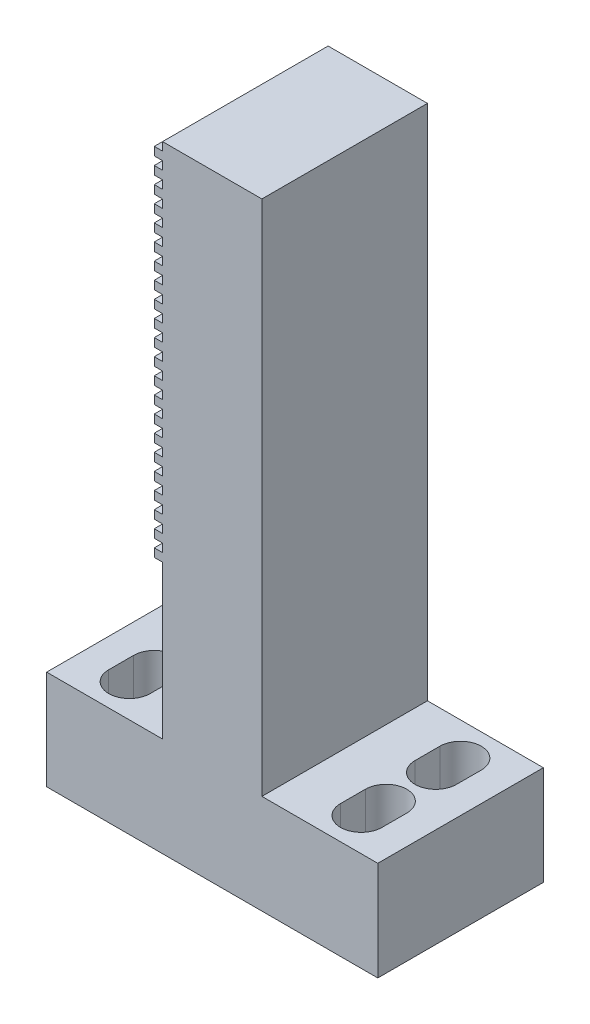
from build123d import *

# Parameters (mm, degrees)
EXTRUDE_1_DEPTH        = 10
CUT_EXTRUDE_1_REACH    = 68.38
SKETCH_3_W             = 20
SKETCH_3_H             = 1
EXTRUDE_2_DEPTH        = 1
PATTERN_LINEAR_1_COUNT = 22
PATTERN_LINEAR_1_PITCH = 2


with BuildPart() as part:
    # 草图1 → 凸台-拉伸1 (new, symmetric)
    with BuildSketch(Plane.XY):
        Polygon((0, 0), (-20, 0), (-20, 12), (-6, 12), (-6, 74.5), (6, 74.5), (6, 12), (20, 12), (20, 0), align=None)
    extrude(amount=EXTRUDE_1_DEPTH, both=True)

    # 草图2 → 切除-拉伸1 (cut, up to next)
    with BuildSketch(Plane(origin=(0, 12, 0), x_dir=(1, 0, 0), z_dir=(0, 1, 0)), mode=Mode.PRIVATE) as cut_extrude_1_sk1:
        with BuildLine():
            Line((-16.5, 3), (-16.5, 6))
            ThreePointArc((-16.5, 6), (-14, 8.5), (-11.5, 6))
            Line((-11.5, 6), (-11.5, 3))
            ThreePointArc((-11.5, 3), (-14, 0.5), (-16.5, 3))
        make_face()
    cut_extrude_1_tool1 = extrude(cut_extrude_1_sk1.sketch, amount=-CUT_EXTRUDE_1_REACH, mode=Mode.PRIVATE) & part.part
    # 草图2 → 切除-拉伸1 (cut, up to next)
    with BuildSketch(Plane(origin=(0, 12, 0), x_dir=(1, 0, 0), z_dir=(0, 1, 0)), mode=Mode.PRIVATE) as cut_extrude_1_sk2:
        with BuildLine():
            Line((-16.5, -6), (-16.5, -3))
            ThreePointArc((-16.5, -3), (-14, -0.5), (-11.5, -3))
            Line((-11.5, -3), (-11.5, -6))
            ThreePointArc((-11.5, -6), (-14, -8.5), (-16.5, -6))
        make_face()
    cut_extrude_1_tool2 = extrude(cut_extrude_1_sk2.sketch, amount=-CUT_EXTRUDE_1_REACH, mode=Mode.PRIVATE) & part.part
    # 草图2 → 切除-拉伸1 (cut, up to next)
    with BuildSketch(Plane(origin=(0, 12, 0), x_dir=(1, 0, 0), z_dir=(0, 1, 0)), mode=Mode.PRIVATE) as cut_extrude_1_sk3:
        with BuildLine():
            Line((16.5, -6), (16.5, -3))
            ThreePointArc((16.5, -3), (14, -0.5), (11.5, -3))
            Line((11.5, -3), (11.5, -6))
            ThreePointArc((11.5, -6), (14, -8.5), (16.5, -6))
        make_face()
    cut_extrude_1_tool3 = extrude(cut_extrude_1_sk3.sketch, amount=-CUT_EXTRUDE_1_REACH, mode=Mode.PRIVATE) & part.part
    # 草图2 → 切除-拉伸1 (cut, up to next)
    with BuildSketch(Plane(origin=(0, 12, 0), x_dir=(1, 0, 0), z_dir=(0, 1, 0)), mode=Mode.PRIVATE) as cut_extrude_1_sk4:
        with BuildLine():
            Line((16.5, 3), (16.5, 6))
            ThreePointArc((16.5, 6), (14, 8.5), (11.5, 6))
            Line((11.5, 6), (11.5, 3))
            ThreePointArc((11.5, 3), (14, 0.5), (16.5, 3))
        make_face()
    cut_extrude_1_tool4 = extrude(cut_extrude_1_sk4.sketch, amount=-CUT_EXTRUDE_1_REACH, mode=Mode.PRIVATE) & part.part
    add(cut_extrude_1_tool1.solids().sort_by_distance((-14, 12, -4.5))[0], mode=Mode.SUBTRACT)
    add(cut_extrude_1_tool2.solids().sort_by_distance((-14, 12, 4.5))[0], mode=Mode.SUBTRACT)
    add(cut_extrude_1_tool3.solids().sort_by_distance((14, 12, 4.5))[0], mode=Mode.SUBTRACT)
    add(cut_extrude_1_tool4.solids().sort_by_distance((14, 12, -4.5))[0], mode=Mode.SUBTRACT)

    # 草图3 → 凸台-拉伸2 (add)
    with BuildSketch(Plane.ZY.offset(6)):
        with Locations((0, 73)):
            Rectangle(SKETCH_3_W, SKETCH_3_H)
    extrude_2 = extrude(amount=EXTRUDE_2_DEPTH)

    # 阵列(线性)1: 凸台-拉伸2 ×22
    with Locations(*[(0, -i * PATTERN_LINEAR_1_PITCH, 0) for i in range(1, PATTERN_LINEAR_1_COUNT)]):
        add(extrude_2)


solid = part.part
